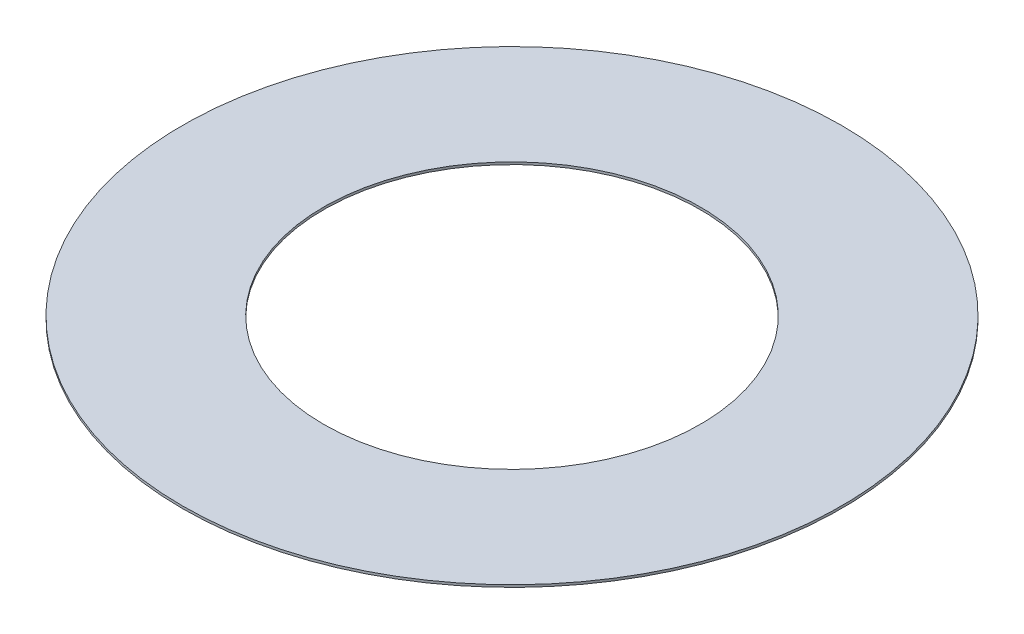
from build123d import *

# Parameters (mm, degrees)
SKETCH1_R           = 7
SKETCH1_R_2         = 4
BOSS_EXTRUDE1_DEPTH = 0.05


with BuildPart() as part:
    # Sketch1 → Boss-Extrude1 (new body)
    with BuildSketch(Plane(origin=(0, 0, 0), x_dir=(1, 0, 0), z_dir=(0, 1, 0))):
        with Locations(Location((0, 0, 0), (0, 0, 270))):
            Circle(SKETCH1_R)
        with Locations(Location((0, 0, 0), (0, 0, 270))):
            Circle(SKETCH1_R_2, mode=Mode.SUBTRACT)
    extrude(amount=BOSS_EXTRUDE1_DEPTH)


solid = part.part
